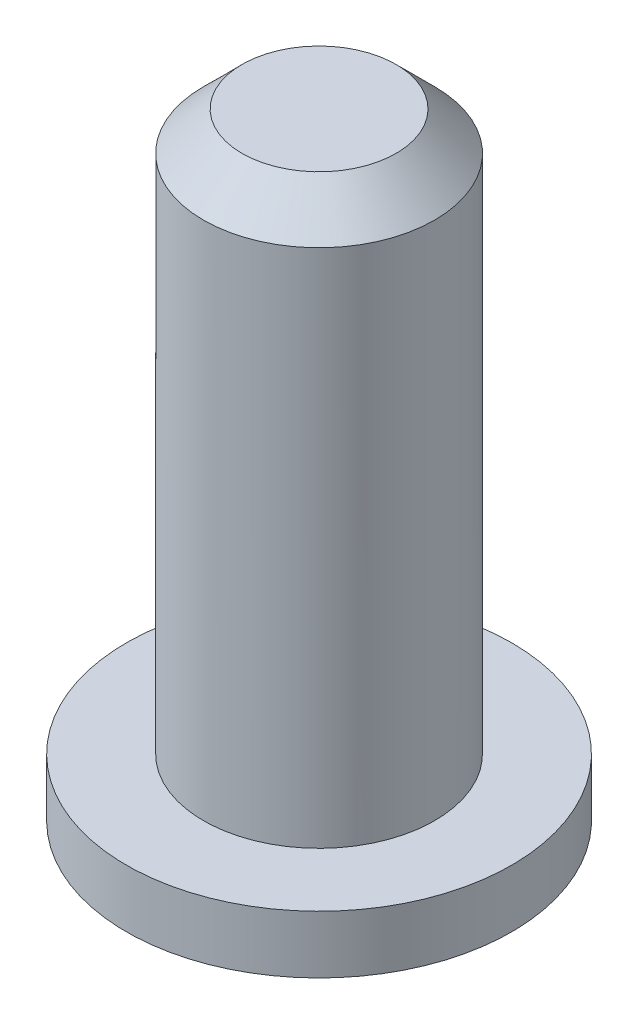
SolidWorks part; units mm, degrees
ref_plane "Front Plane" through (0, 0, 0) normal (0, 0, 1) x (1, 0, 0)
ref_plane "Top Plane" through (0, 0, 0) normal (0, 1, 0) x (1, 0, 0)
ref_plane "Right Plane" through (0, 0, 0) normal (1, 0, 0) x (0, 0, -1)
sketch "Sketch1" plane through (0, 0, 0) normal (0, 0, 1) x (1, 0, 0)
  line L0 (0, 0) -> (0, 138.3939) construction
  line L1 (0, 0) -> (10, 0)
  line L2 (10, 0) -> (10, 3)
  line L3 (10, 3) -> (6, 3)
  line L4 (6, 3) -> (6, 32)
  line L5 (6, 32) -> (0, 32)
  line L6 (0, 32) -> (0, 0)
  dimension "D1" = 6
  dimension "D2" = 10
  dimension "D3" = 32
  dimension "D4" = 3
revolve "Revolve1" add sketch "Sketch1" angle 360 about L0
chamfer "Chamfer1" distance 2 angle 45 1 edges at (0, 32, -6)
